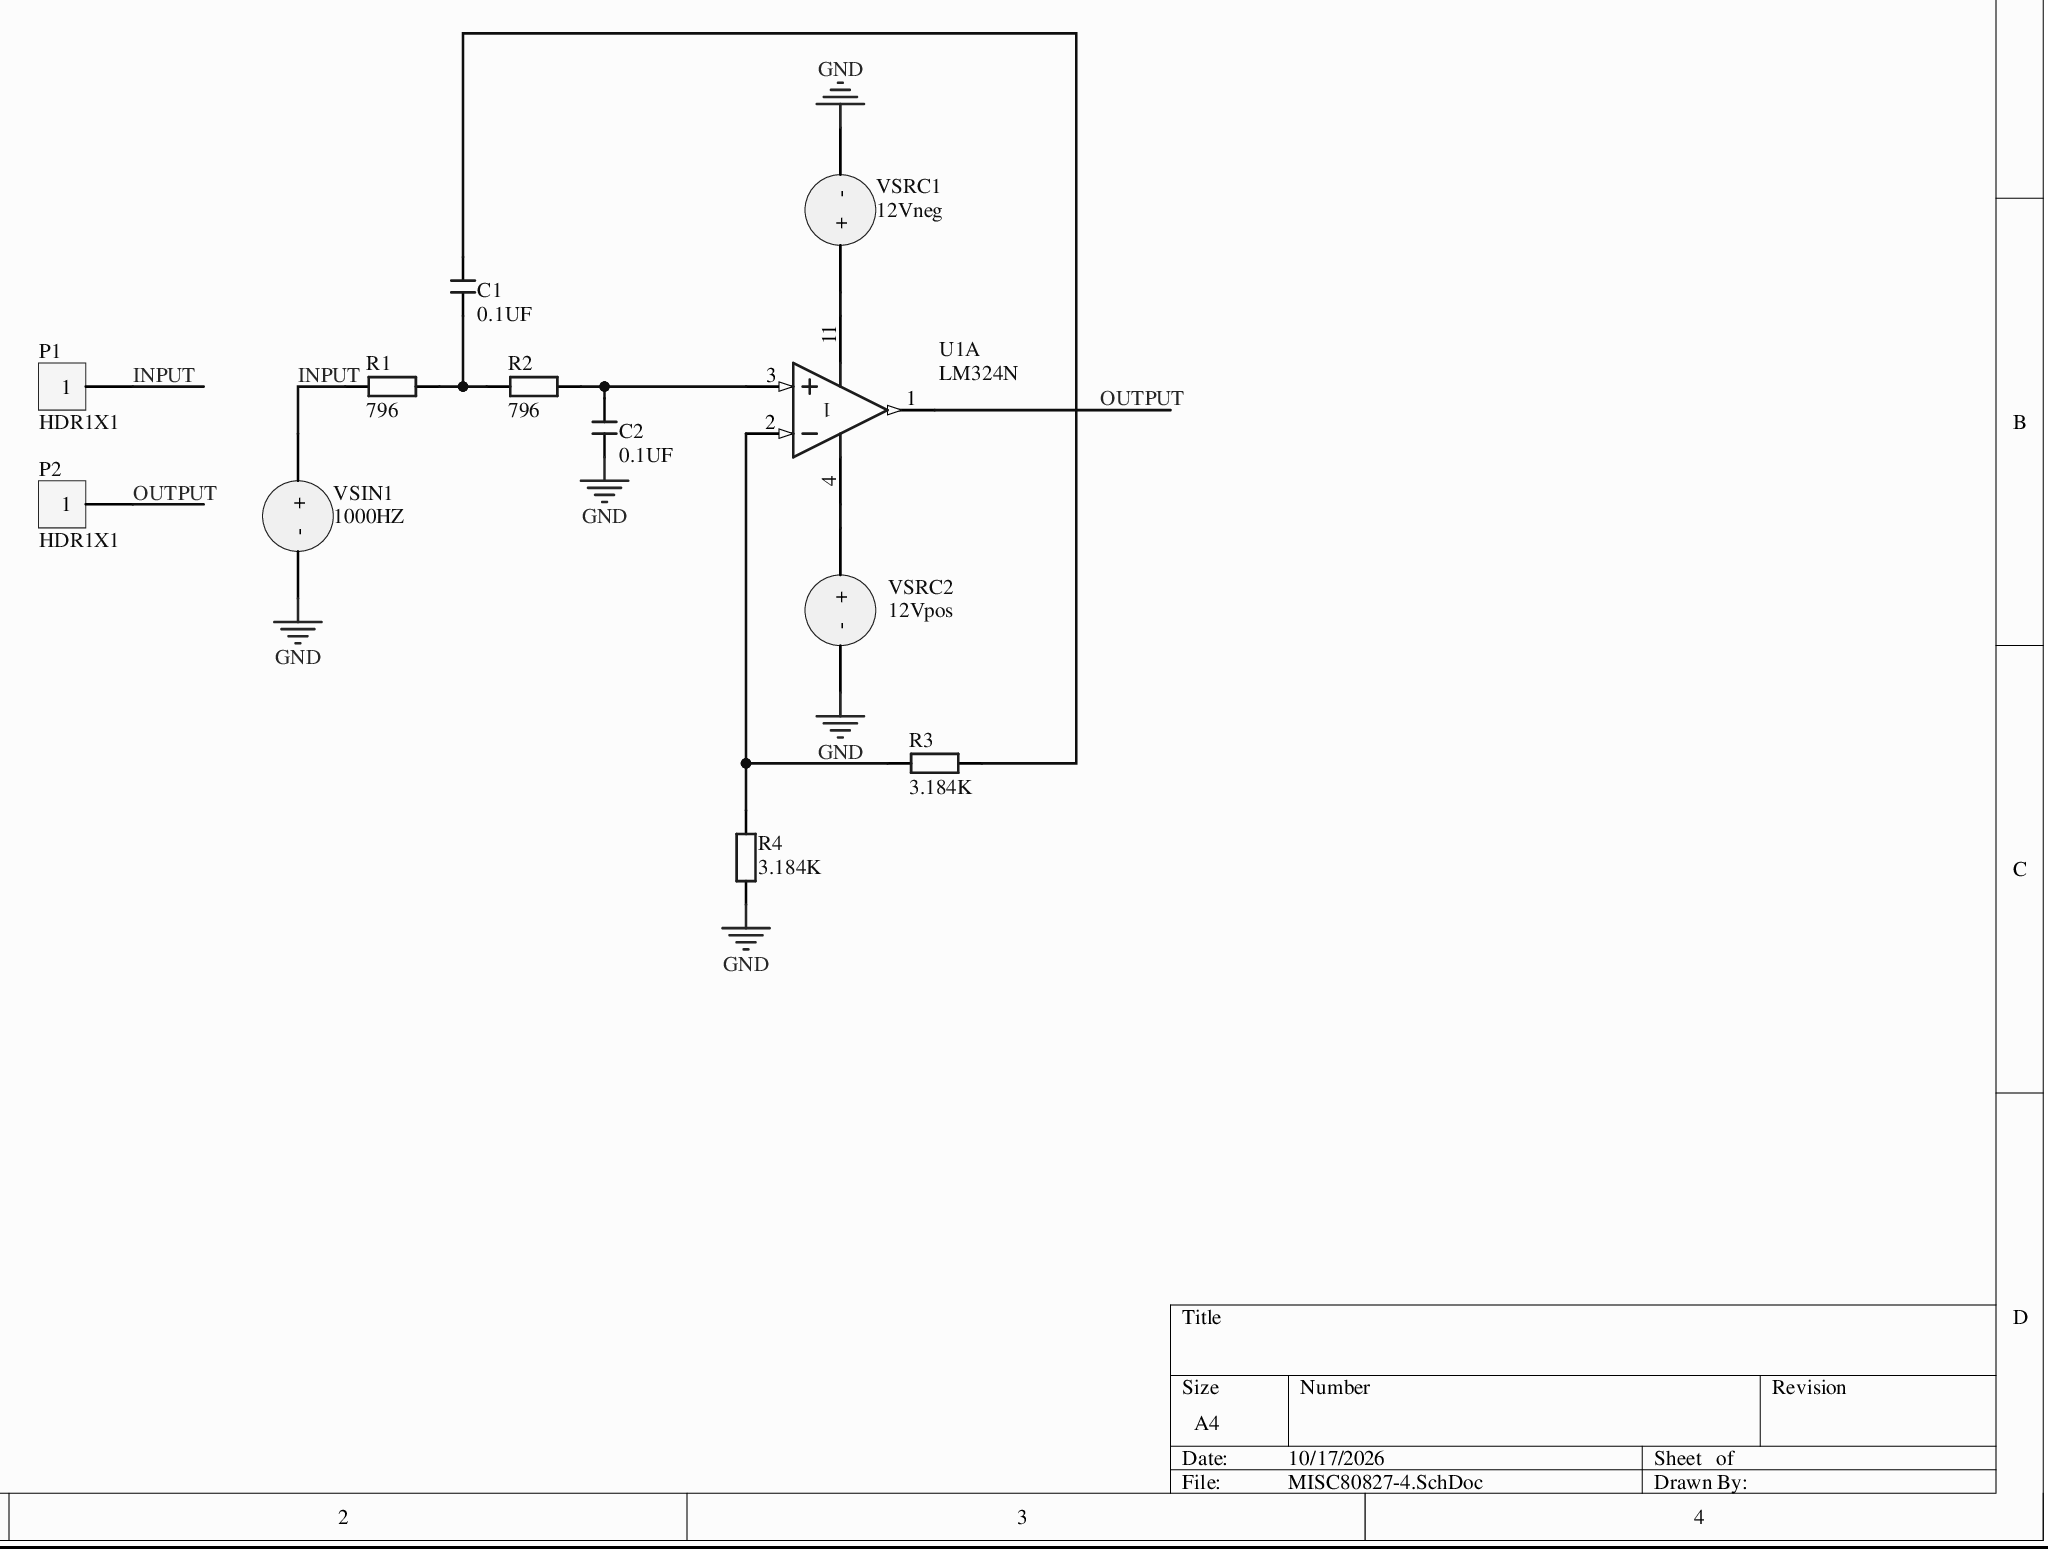
[diagram p0: MISC80827-4.SchDoc]
# Altium project MISC80827-7.PrjPcb
1 sheet, 12 parts. Net scope: global (net labels, ports and power ports of the same name join across sheets).
Board file: MISC80827.PcbDoc

## Sheet MISC80827-4.SchDoc
size A4

### Parts
C1  0.1UF  [MLCC5.08-A]
C2  0.1UF  [MLCC5.08-A]
P1  HDR1X1  [HDR1X1]
P2  HDR1X1  [HDR1X1]
R1  796  [RS 1/4W]
R2  796  [RS 1/4W]
R3  3.184K  [RS 1/4W]
R4  3.184K  [RS 1/4W]
U1  LM324N  [646-06]  (part A of 4)
VSIN1  1000HZ  [HDR1X2]
VSRC1  12Vneg  [HDR1X2]
VSRC2  12Vpos  [HDR1X2]

### Nets
GND: C2.1 R4.1 VSIN1.2(-) VSRC1.2(-) VSRC2.2(-)
INPUT: P1.1 R1.1 VSIN1.1(+)
OUTPUT: P2.1 U1.1(OUT)
NetC1_1: C1.1 R1.2 R2.1
NetC1_2: C1.2 R3.1
NetC2_2: C2.2 R2.2 U1.3(IN+)
NetR3_2: R3.2 R4.2 U1.2(IN-)
NetU1_4: U1.4(V+) VSRC2.1(+)
NetU1_11: U1.11(V-) VSRC1.1(+)

### Library data of the parts
C1 C2 = C-MLCC: Monolithic ceramic capacitor; BOM名称: Monolithic ceramic capacitor
R1-R4 = R-S: Color-band resistor; BOM名称: Color-band resistor
U1 = LM324N: Quad Low-Power Operational Amplifier; Package Information: Latest Revision: 1997; Published: 17-Jul-2002; Datasheet: Linear and Interface Integrated Circuits, DL128 Rev2 (1988); Package Reference: 646-06; Publisher: Altium Limited
VSIN1 VSRC1 VSRC2 = 电流源